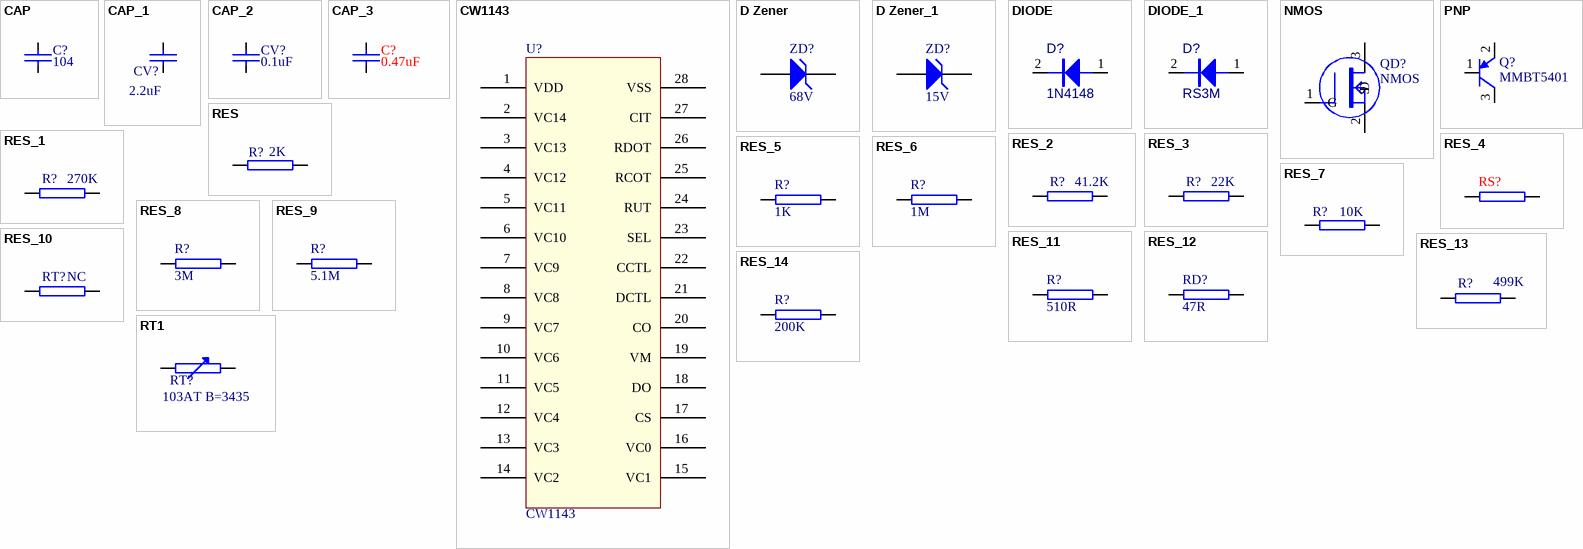
[diagram p0: symbols CAP to RT1]
# Altium schematic symbol library MISC84391-4.SchLib: 27 symbols
Pins are listed as number, name and electrical type; pins without a type are passive.


## CAP
designator C?, comment 104
footprint 0603
footprint 0603C
footprint CAP0603 (CAP0402)
pins: 1, 2

## CAP_1
designator CV?, comment 2.2uF
footprint 0805C
footprint CAP0603 (CAP0402)
footprint CAP0805
pins: 1, 2

## CAP_2
designator CV?, comment 0.1uF
footprint 0603C
footprint CAP0603
pins: 1, 2

## CAP_3
designator C?, comment 0.47uF
footprint 0603C
footprint CAP0603 (CAP0402)
pins: 1, 2

## CW1143
designator U?
footprint SSOP-28-0.635 (Footprint not found)
pins: 1 VDD, 2 VC14, 3 VC13, 4 VC12, 5 VC11, 6 VC10, 7 VC9, 8 VC8, 9 VC7, 10 VC6, 11 VC5, 12 VC4, 13 VC3, 14 VC2, 15 VC1, 16 VC0, 17 CS, 18 DO, 19 VM, 20 CO, 21 DCTL, 22 CCTL, 23 SEL, 24 RUT, 25 RCOT, 26 RDOT, 27 CIT, 28 VSS

## D Zener
designator ZD?, comment 68V
Zener Diode
footprint SOD123
simulation model ZENER (Diode)
signal-integrity model D Zener
pins: 1 A, 2 K

## D Zener_1
designator ZD?, comment 15V
Zener Diode
footprint SOD323
simulation model ZENER (Diode)
signal-integrity model D Zener
pins: 1 A, 2 K

## DIODE
designator D?, comment 1N4148
DIODE
footprint DIODE0.4
footprint DIODE0.1
footprint DIODE0.3
footprint DIODE0.5
footprint SOD323
pins: 1 A, 2 K
2 alternate drawings of the same symbol

## DIODE_1
designator D?, comment RS3M
DIODE
footprint DIODE0.4
footprint DIODE0.1
footprint DIODE0.3
footprint DIODE0.5
footprint SMC
pins: 1 A, 2 K
2 alternate drawings of the same symbol

## NMOS
designator QD?
footprint SOT-23-3
footprint TO-252
footprint to-252-A
footprint TO-252-A
footprint TO-252-A
footprint TOLL
footprint TO-263
footprint TO-263-TOLL
footprint TOLL_123 (SMD MOSFET)
pins: 1 G, 2 S, 3 D

## PNP
designator Q?, comment MMBT5401
PNP Bipolar Transistor
footprint SOT-23B_N (SOT23, 3-Leads, Body 2.9x1.3mm, Pitch 0.95mm, Lead Span 2.4mm, IPC Medium Density)
footprint SOT-23B_L (SOT23, 3-Leads, Body 2.9x1.3mm, Pitch 0.95mm, Lead Span 2.4mm, IPC High Density)
footprint SOT-23B_M (SOT23, 3-Leads, Body 2.9x1.3mm, Pitch 0.95mm, Lead Span 2.4mm, IPC Low Density)
simulation model PNP
signal-integrity model PNP
footprint SOT-23-3
pins: 1 B, 2 E, 3 C

## RES
designator R?, comment 2K
footprint 0603
footprint RES0805
pins: 1, 2

## RES_1
designator R?, comment 270K
footprint 0603
footprint 0603R
footprint RES0603
pins: 1, 2

## RES_2
designator R?, comment 41.2K
footprint 0603
footprint 0603R
footprint RES0603
pins: 1, 2

## RES_3
designator R?, comment 22K
footprint 0603
footprint 0603R
footprint RES0603
pins: 1, 2

## RES_4
designator RS?
footprint 0603
footprint 2512
pins: 1, 2

## RES_5
designator R?, comment 1K
footprint 0603
footprint 0603R
footprint RES0603
pins: 1, 2

## RES_6
designator R?, comment 1M
footprint 0603
footprint 0603R
footprint RES0603
pins: 1, 2

## RES_7
designator R?, comment 10K
footprint 0603
footprint 0603R
footprint RES0603
pins: 1, 2

## RES_8
designator R?, comment 3M
footprint 0603
footprint 0603R
footprint RES0603
pins: 1, 2

## RES_9
designator R?, comment 5.1M
footprint 0603
footprint 0603R
footprint RES0603
pins: 1, 2

## RES_10
designator RT?, comment NC
footprint 0603
footprint 0603R
footprint RES0603
pins: 1, 2

## RES_11
designator R?, comment 510R
footprint 0603
footprint 0603R
footprint RES0603
pins: 1, 2

## RES_12
designator RD?, comment 47R
footprint 0603
footprint 0603R
footprint RES0603
pins: 1, 2

## RES_13
designator R?, comment 499K
footprint 0603
footprint 0603R
footprint RES0603
pins: 1, 2

## RES_14
designator R?, comment 200K
footprint 0603
footprint 0603R
footprint RES0603
pins: 1, 2

## RT1
designator RT?, comment 103AT B=3435
footprint WK
pins: 1, 2